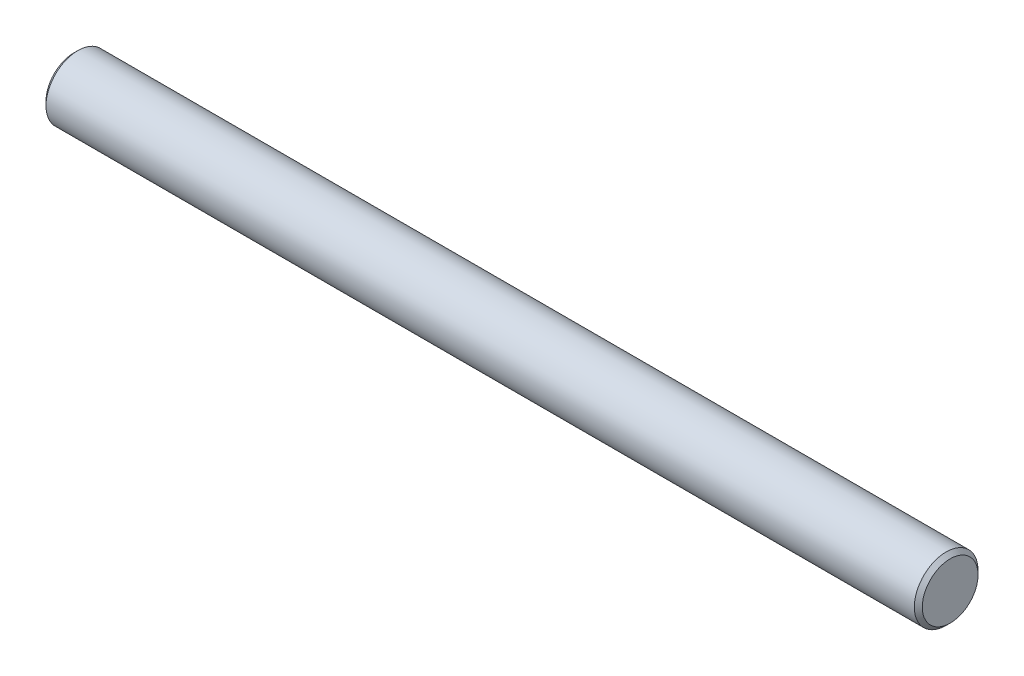
SolidWorks part; units mm, degrees
material "镀铬棒"
ref_plane "Front Plane" through (0, 0, 0) normal (0, 0, 1) x (1, 0, 0)
ref_plane "Top Plane" through (0, 0, 0) normal (0, 1, 0) x (1, 0, 0)
ref_plane "Right Plane" through (0, 0, 0) normal (1, 0, 0) x (0, 0, -1)
sketch "Sketch1" plane through (0, 0, 0) normal (0, 0, 1) x (1, 0, 0)
  line L0 (0, 0) -> (110, 0) construction
  line L1 (0, 0) -> (0, 4)
  line L2 (0, 4) -> (110, 4)
  line L3 (110, 4) -> (110, 0)
  line L4 (0, 0) -> (110, 0)
  dimension "D1" = 8
  dimension "D2" = 110
revolve "Revolve1" add sketch "Sketch1" angle 360 about L0
sketch "Sketch2" plane through (0, 0, 0) normal (0, 1, 0) x (1, 0, 0)
  line L0 (110, 4) -> (0, 4) construction
  line L1 (2, 3) -> (6, 3)
  line L2 (2, 3) -> (2, 5)
  line L3 (2, 5) -> (6, 5)
  line L4 (6, 3) -> (6, 5)
  line L5 (2, 3) -> (6, 5) construction
  line L6 (2, 5) -> (6, 3) construction
  line L7 (0, 4) -> (0, -4) construction
  line L8 (110, 4) -> (0, 4) construction
  point P0 (4, 4)
  dimension "D1" = 4
  dimension "D2" = 4
  dimension "D3" = 1
extrude "Cut-Extrude1" cut sketch "Sketch2" against normal mid plane 10
chamfer "Chamfer1" distance 0.5 angle 45 2 edges at (110, 0, 4) (0, 0, 4)
